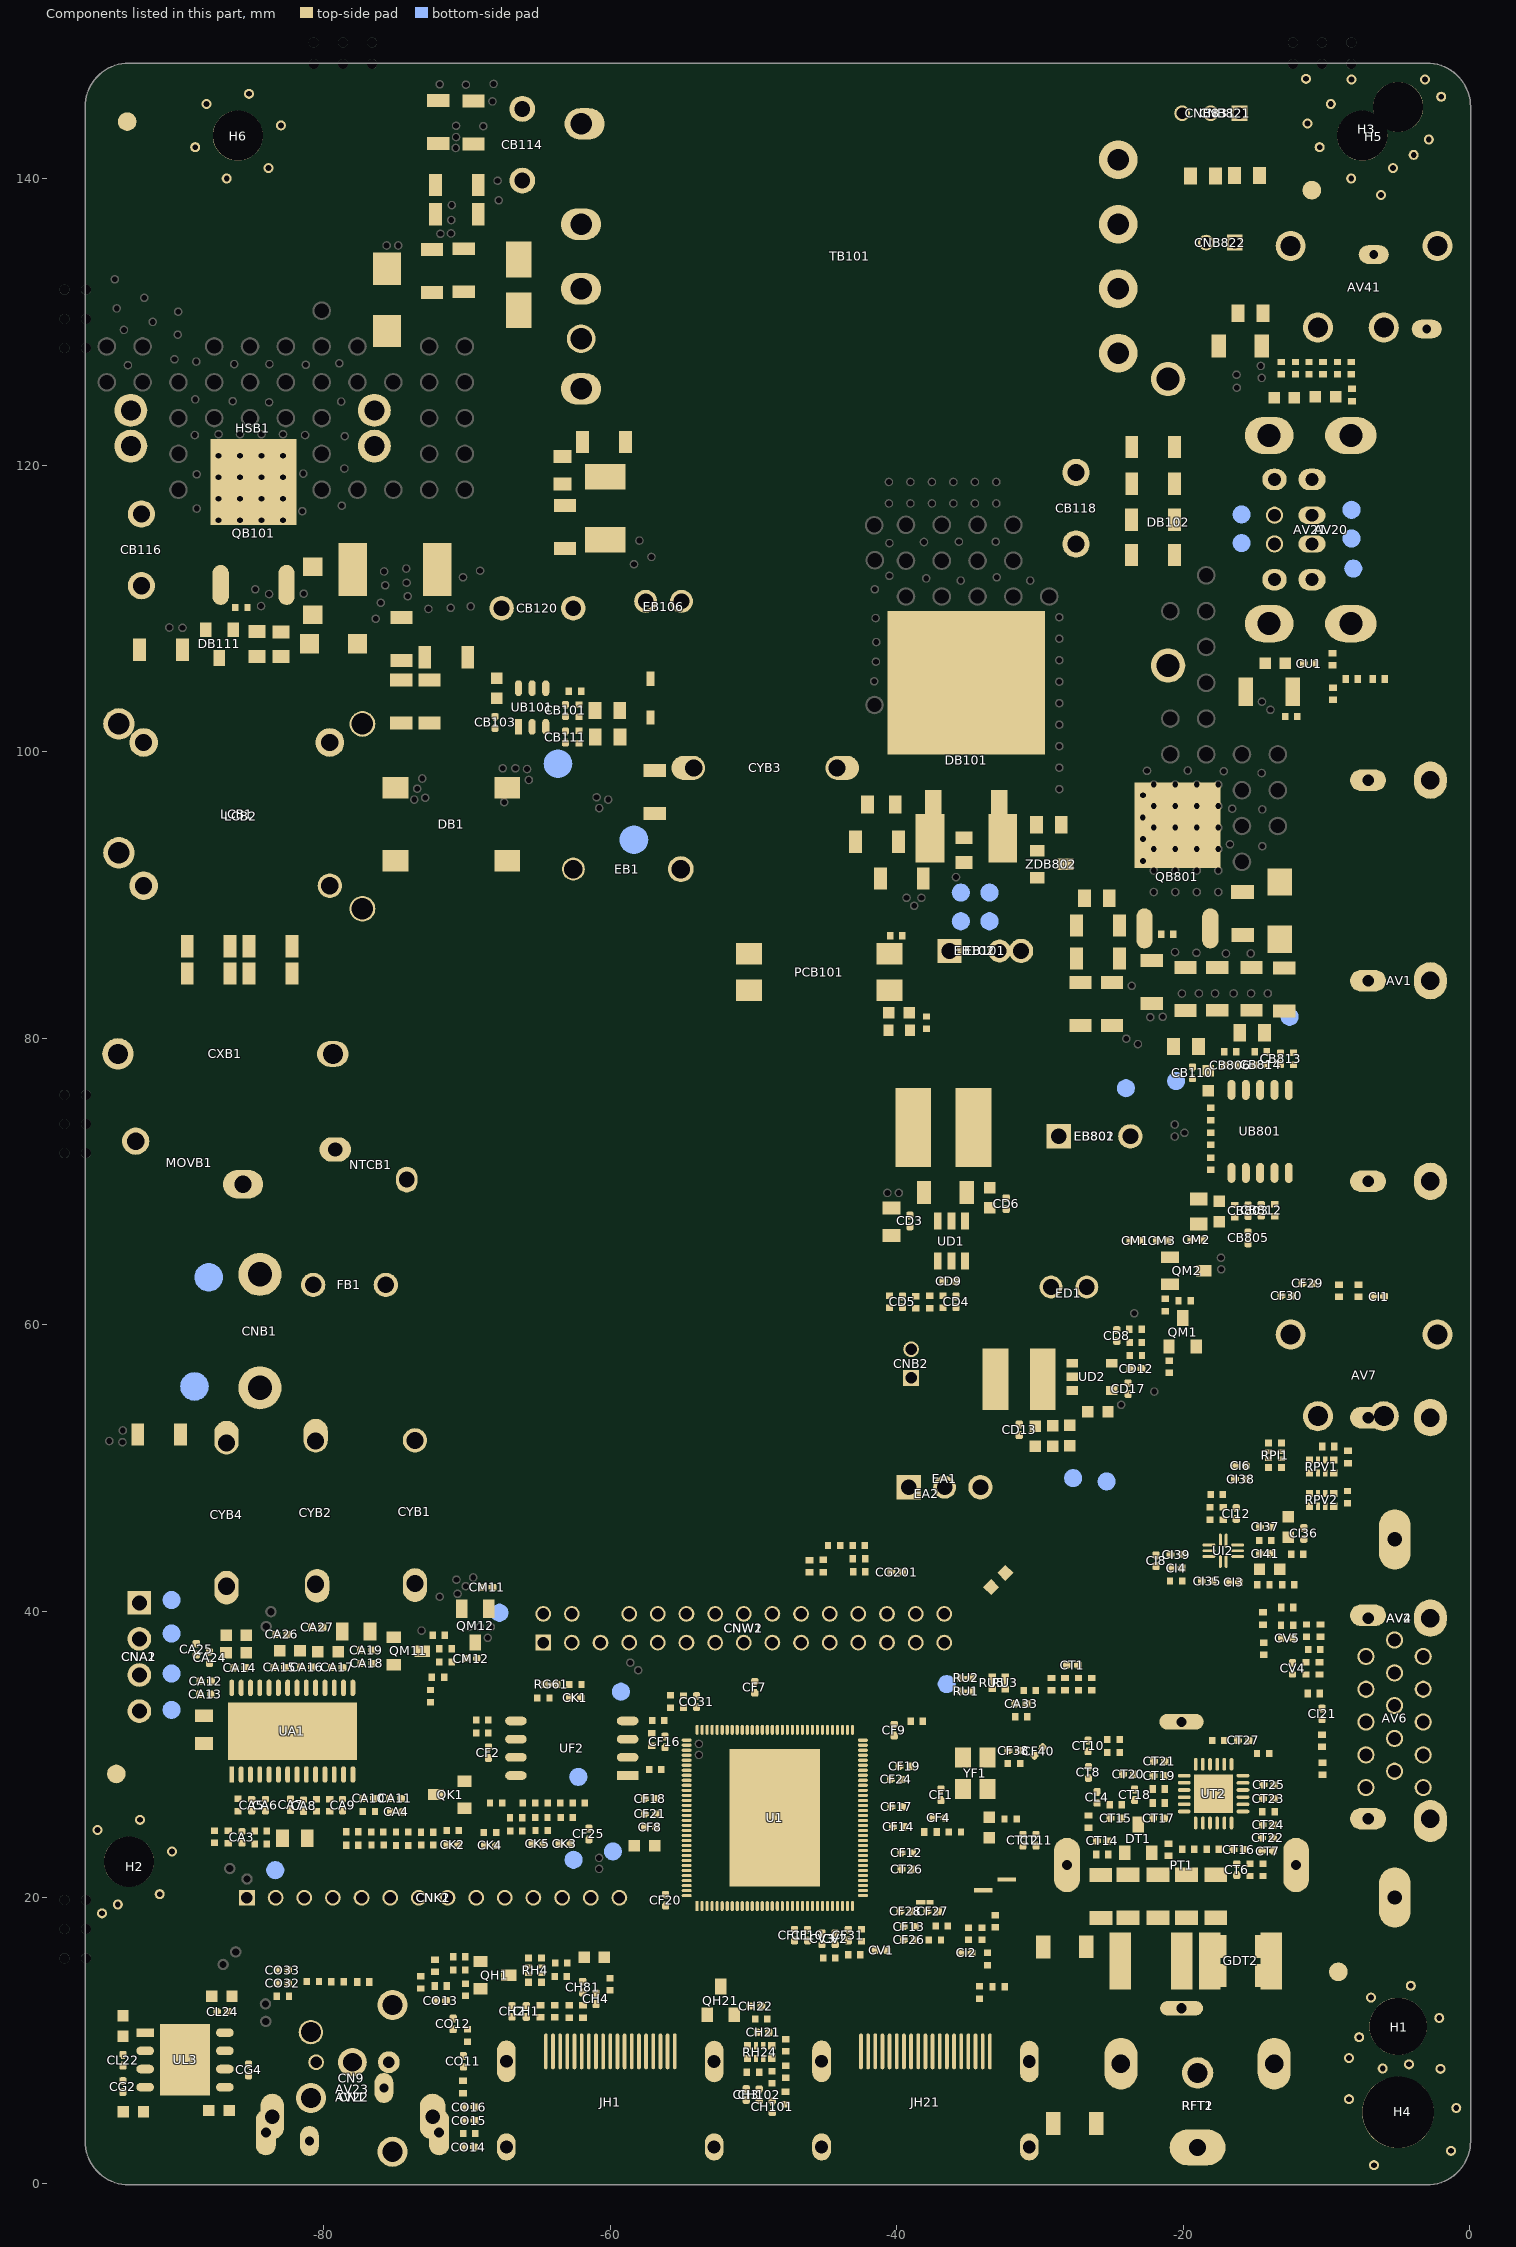
[diagram p0: the components of this part, seen from the top]
# Altium PCB MISC86372.PcbDoc (part 16 of 16)
Units mm, origin at the board's own origin, x right, y up, seen from the top; angles counter-clockwise.
Board outline 96.73 x 148.13 mm, 2 copper layers (TopLayer, BottomLayer), stack 1.571 mm thick; 578 components, 318 nets, 2702 pads, 836 vias.

## Silkscreen, mask and mechanical layers (free items; w line width, h text height)
TopOverlay:
  drawing of 502 lines, arcs and shapes, not listed
  text "2" at -3.2,226.609 h4.06
  text "3" at -191.5,220.391 h4.06 r180
  text "Solder Mask:" at 150.475,177.774 h1.52
  text "IPC SM-840" at 160.952,177.749 h1.52
  text "Silkscreen Color:" at 180.409,177.749 h1.52
  text "White" at 192.575,177.749 h1.52
  text "Units:" at 180.409,175.234 h1.52
  text "PTH Copper Thickness:" at 150.475,175.209 h1.52
  text ">20um" at 167.582,175.184 h1.52
  text "mm" at 185.438,175.196 h1.52
  text "Dielectric Constant Er@1GHz To 1MHz:" at 150.466,172.695 h1.52
  text "4.2 --- 4.6" at 180.425,172.708 h1.52
  text "Panel Size:" at 150.424,170.193 h1.52
  text "2L,4,97.35×148.75mm,FR4(TG130-CTI175),1OZ,Green,OSP,1.2mm" at 158.175,170.193 h1.52
  text "Silkscreen on PTH:" at 150.437,167.614 h1.52
  text "Primary Side Retained;" at 163.594,167.589 h1.52
  text "Secondary Side  Removed for Soldering" at 180.409,167.551 h1.52
  text "Special Requirements" at 150.411,165.311 h1.52
  text "If engineering questions are not answered within 2 hours, call PHONE_A" at 198.332,165.126 h1.52
  text "1. Lead-free HASL (HAL_LF, Lead Free Hot Air Leveling)" at 165.42,162.68 h1.52
  text "2. OSP (OSP, Organic Solderability Preservatives)" at 165.42,160.546 h1.52
  text "3. ENIG (ENIG, Electroless Nickel/Immersion Gold)" at 165.382,158.222 h1.52
  text "Plated Technics" at 152.316,157.34 h1.52
  text "4. ENIG + gold finger (ENIG_G/F, Electroless Nickel/Immersion Gold + Gold Finger)" at 165.42,156.178 h1.52
  text "5. Gold plating (Gold_plated, Gold-plated)" at 165.445,154.133 h1.52
  text "6. Gold plating + gold finger (Gold_Plated_G/F, Gold-plated + Gold Finger)" at 165.458,152.152 h1.52
  text "LED DRIVER" at -30.785,146.634 h1.52
  text "Impedance Control" at 150.532,146.345 h1.52
  text "Target Impedance" at 170.771,146.348 h1.52
  text "Layer(s)" at 209.23,146.35 h1.52
  text "Width & Clearance" at 189.715,146.342 h1.52
  text "75 +/- 10% Ohm" at 171.335,143.79 h1.52
  text "G/12/15.8/12/G mil" at 188.634,143.773 h1.52
  text "layer 1" at 209.23,143.776 h1.52
  text "Single End Impedance" at 150.532,142.616 h1.52
  text "75 +/- 10% Ohm" at 171.335,141.301 h1.52
  text "G/6.2/7.1/6.2/G mil" at 188.634,141.284 h1.52
  text "layer 1&2" at 209.23,141.287 h1.52
  text "[ Zo ]" at 156.208,139.13 h1.52
  text "G/5/7/5/7/5/G mil" at 188.888,133.841 h1.52
  text "100 +/- 10% Ohm" at 171.005,133.816 h1.52
  text "layer 1" at 209.509,133.771 h1.52
  text "Differential Impedance" at 150.528,132.416 h1.52
  text "9/4/9 mil" at 188.838,131.322 h1.52
  text "100 +/- 10% Ohm" at 170.955,131.297 h1.52
  text "layer 1" at 209.46,131.251 h1.52
  text "[ Zo ]" at 156.196,129.283 h1.52
  text "( G: Ground )" at 153.912,126.553 h1.52
  text "90 +/- 10% Ohm" at 171.666,126.247 h1.52
  text "layer 1" at 209.408,126.227 h1.52
  text "G/5/11/5/11/5/G mil" at 188.888,126.158 h1.52
  text "Common Mode Impedance" at 150.014,120.922 h1.52
  text "[ Zc ]" at 156.314,118.865 h1.52
  text "Refer to Gerber documents GTP&GBP for Stencil aperture design" at 173.257,112.154 h1.52
  text "Stencil" at 150.377,109.69 h1.52
  text "NEW" at 173.203,107.213 h1.52
  text "Test jig" at 150.329,104.721 h1.52
  text "The Same As XXXXXXXXXXXXXX XXXXXX" at 173.234,104.696 h1.52
  text "Wave-soldering jig" at 150.385,102.226 h1.52
  text "The Same As XXXXXXXXXXXXXX XXXXXX" at 173.285,102.055 h1.52
  text "Solder paste" at 173.194,99.64 h1.52
  text "Production process" at 150.346,99.602 h1.52
  text "[Process and notes]" at 154.924,97.447 h1.52
  text "Stencil at HDMI is cut to the actual pattern" at 173.304,97.409 h1.52
  text "Only one barcode position on the board; the other barcode must be attached to a component" at 192.075,97.409 h1.52
  text "Special requirements" at 150.372,94.573 h1.52
  text "SMD components over 2mm high on the wave-soldering side" at 150.365,91.999 h1.52
  text "Packaging notes" at 150.356,89.555 h1.52
  text "[Fragile components]" at 156.486,87.402 h1.52
  text "Footprint matching" at 150.356,84.475 h1.52
  text "[New component footprint]" at 156.13,82.347 h1.52
  text "(Automated Testing Support)" at 158.442,79.439 h1.14
  text "Automated test support" at 150.352,79.35 h1.52
  text "NO" at 174.919,78.064 h1.52
  text "[Reserved suction cup and press bar positions]" at 154.429,77.204 h1.52
  text "1" at -3.168,77.109 h4.06
  text "4" at -191.5,70.891 h4.06 r180
  text "Layer Stack Up Detail for" at 153.936,68.072 h2.54
  text ".Pcb_File_Name_No_Path" at 180.881,68.072 h2.54
  text "Layer" at 158.111,64.319 h1.27
  text "Gerber" at 167.552,64.319 h1.27
  text "Layer" at 175.455,64.319 h1.27
  text "Layer" at 191.616,64.319 h1.27
  text "Copper" at 211.654,64.319 h1.27
  text "Dielectric" at 219.573,64.319 h1.27
  text "Stack up" at 191.616,63.027 h1.27
  text "Height" at 219.573,63.027 h1.27
  text "Name" at 158.111,62.989 h1.27
  text "Document" at 167.552,62.989 h1.27
  text "Ordor" at 175.455,62.989 h1.27
  text "Thickness" at 211.654,62.989 h1.27
  text "12V" at -34.679,58.546 h1.27 r90
  text "TopOverlay" at 158.103,57.074 h1.52
  text ".GTO" at 168.506,57.009 h1.52
  text "PWR UPGRADE" at -41.614,56.411 h1.52 r90
  text "GND" at -34.699,54.948 h1.27 r90
  text "0.4mil" at 219.505,54.85 h1.52
  text "1" at 176.807,52.23 h1.52
  text "1.4mil" at 211.986,52.228 h1.52
  text "2" at 176.808,46.818 h1.52
  text "1.4mil" at 211.942,46.793 h1.52
  text "0.4mil" at 219.573,44.388 h1.52
  text "LVDS" at -61.109,42.924 h1.52
  text "Notes:" at 149.768,30.091 h2.03
  text "1. No Plated Through Hole  overlap each other should be combined ,Residues between them should be eliminated." at 149.746,27.858 h1.52
  text "SPEAKER" at -93.142,26.797 h1.52
  text "2. Plated Through Hole superposition should be made as a bigger one." at 149.745,25.925 h1.52
  text "3. When there is not enough space for UL authentication marking,Manufacturer ID code and the Bar Code frame," at 149.746,24.185 h1.52
  text "only the Manufacturer  ID code is needed and layed wherever it can be." at 151.229,22.39 h1.52
  text "4. Spacing between two pads of IC package should be covered with solder oil." at 149.746,20.44 h1.52
  text "5. All trace should be covered with green oil unless otherwise specified. If discovers unusually, please confirm with us." at 149.746,18.575 h1.52
  text "KEY&IR&LED" at -88.468,17.704 h1.52 r90
  text "6. Silkscreen overlaped SMD pads should be removed directly." at 149.746,16.713 h1.52
  text "7. The width of Carbon Sprayed must be 16mil wider than its trace." at 149.746,14.909 h1.52
  text "8. Bridging Thickness of V-cut  should be kept within 0.3±0.1mm when the width of single piece bare board is smaller than 20mm." at 149.746,13.018 h1.52
  text "9. There is no need to plugged with green oil when the diameter of vias is bigger than 0.6mm." at 149.746,10.94 h1.52
  text "10. All vias under BGA must be covered and plugged with Solder oil." at 149.747,8.911 h1.52
BottomOverlay:
  drawing of 153 lines, arcs and shapes, not listed
  text "+" at -15.697,146.069 h2
  text "-" at -19.676,145.949 h3
  text "-" at -17.676,145.949 h3
  text "EARPHONE OUT" at -1.064,137.184 h1.52
  text "+" at -15.799,137.135 h2
  text "-" at -17.907,137.008 h3
  text "USB2 IN" at -3.967,111.681 h1.52 r270
  text "USB1 IN" at -1.986,111.656 h1.52 r270
  text "AV IN / YPBPR AUDIO IN" at -5.436,69.723 h1.52 r270
  text "FB1" at -71.501,59.766 h1.27
  text "PC AUDIO IN" at -1.408,56.142 h1.52
  text ".GBO" at 168.547,41.934 h1.52
  text "BottomOverlay" at 157.837,41.909 h1.52
  text "VGA IN" at -2.393,18.128 h1.52 r270
  text "K7" at -83.795,17.018 h1.27 r270
  text "K6" at -81.661,17.018 h1.27 r270
  text "K5" at -79.681,17.018 h1.27 r270
  text "K4" at -77.755,17.018 h1.27 r270
  text "K3" at -75.717,17.018 h1.27 r270
  text "K2" at -73.681,17.018 h1.27 r270
  text "K1" at -71.653,17.018 h1.27 r270
  text "K0" at -69.647,17.018 h1.27 r270
  text "YPBPR IN" at -8.623,16.897 h1.52 r270
  text "IR" at -65.684,16.79 h1.27 r270
  text "5V" at -59.512,16.637 h1.27 r270
  text "RED" at -61.758,16.129 h1.27 r270
  text "GND" at -67.742,16.027 h1.27 r270
  text "GRN" at -63.729,16.027 h1.27 r270
  text "GND" at -85.979,15.977 h1.27 r270
  text "MINIAV OUT" at -73.076,15.443 h1.52
  text "OPTICAL OUT" at -72.796,14.173 h1.52
  text "RF IN" at -12.733,2.59 h1.52
  text "HDMI2 IN" at -34.77,0.796 h1.52
  text "HDMI1(ARC) IN" at -54.844,0.732 h1.52
  text "COAX/CVBS OUT" at -76.886,0.616 h1.52
TopPaste:
  rectangle: -31.349,4.458 -29.835,5.461
  rectangle: 153.901,58.987 157.208,60.987
  rectangle: -29.184,0.309 -28.94,3.2
  rectangle: -31.342,3.099 -29.82,4.064
  region: -31.342,5.309
  region: -31.342,5.309
  region: -31.349,4.458 -31.346,9.887 -29.116,9.892 -29.116,5.369 -29.83,5.369 -29.83,4.458
  region: -31.333,4.075 -31.3,4.041 -29.852,4.041 -29.852,3.173 -29.857,3.169 -29.851,3.163 -29.156,3.163 -29.156,0.298 -29.162,0.303 -31.327,0.303 -31.327,4.049 -31.342,4.064
  lines w0.127: 167.894,58.987 167.894,60.987 ; 153.901,58.987 172.494,58.987 172.494,60.987 153.901,60.987 153.901,58.987
  lines w0.8: -65.735,93.548 -63.297,95.987
  text "TopPaste" at 158.103,59.526 h1.52
  text ".GTP" at 168.506,59.472 h1.52
BottomPaste:
  rectangle: 153.901,38.983 157.208,40.983
  lines w0.127: 167.894,38.983 167.894,40.983 ; 153.901,38.983 172.494,38.983 172.494,40.983 153.901,40.983 153.901,38.983
  text "BottomPaste" at 157.782,39.567 h1.52
  text ".GBP" at 168.529,39.437 h1.52
TopSolder:
  rectangle: 153.901,54.162 157.208,56.162
  region: -75.87,9.017 -76.302,8.585 -76.302,6.695 -75.982,6.375 -74.905,7.453 -74.905,8.883
  lines w0.127: 167.894,54.162 167.894,56.162 ; 153.901,54.162 172.494,54.162 172.494,56.162 153.901,56.162 153.901,54.162
  lines w0.8: -65.735,93.548 -63.297,95.987
  text "TopSolder" at 158.116,54.673 h1.52
  text ".GTS" at 168.506,54.631 h1.52
BottomSolder:
  drawing of 44 lines, arcs and shapes, not listed
  text "BottomSolder" at 157.782,44.302 h1.52
  text ".GBS" at 168.505,44.279 h1.52
过炉治具:
  drawing of 291 lines, arcs and shapes, not listed
3D和装配:
  circle w0.127: c-9.474,57.988 r15
  circle w0.254: c-24.384,33.246 r25
  circle w0.254: c-8.585,69.977 r25
  circle w0.127: c-7.1,70 r15
  circle w0.127: c-27.4,37.504 r15
  lines w0.127: -5.5,-5.207 -5.5,145 ; -66.747,0.785 -53.247,0.785 -53.247,14.285 -66.747,14.285 -66.747,0.785 ; -44.747,0.785 -31.247,0.785 -31.247,14.285 -44.747,14.285 -44.747,0.785
  text "2L,4,97.35×148.75mm,FR4(TG130-CTI175),1OZ,Green,OSP,1.2mm,5,80,89.4%,1858,0.4mm" at 158.175,170.193 h1.52
自动测试:
  circle w0.152: c-47.409,108.128 r5
  circle w0.152: c-47.38,108.128 r6
  circle w0.152: c-90.179,134.366 r6
  circle w0.152: c-90.208,134.366 r5
顶层限制:
  drawing of 1339 lines, arcs and shapes, not listed
  text "100" at -49.698,167.75 h2.5
  text "89" at -44.198,163.25 h2.5
  text "86" at -42.698,158.75 h2.5
  text "7.5" at -12.856,154.25 h2.5
  text "5" at -2.198,149.75 h2.5
  text "LED DRIVER}" at -51.749,137.101 h3
  text "4-3.5" at -101.544,133.144 h2.5
  text "14" at 11.698,89.217 h2.5 r90
  text "Minimise board expansion}" at -131.258,87.307 h3
  text "14" at 11.743,75.217 h2.5 r90
  text "148" at 51.683,72.75 h2.5 r90
  text "145" at 47.183,71.25 h2.5 r90
  text "143" at 42.683,70.25 h2.5 r90
  text "AC IN}" at -83.133,65.664 h3
  text "132.5" at 38.183,65 h2.5 r90
  text "115.5" at 33.683,56.5 h2.5 r90
  text "LVDS}" at -54.23,46.212 h3
  text "14" at 11.698,44.717 h2.5 r90
  text "84" at 29.183,40.75 h2.5 r90
  text "SPEAKER}" at -88.497,36.189 h3
  text "73.25" at -108.379,35.375 h2.5 r90
  text "14" at 11.743,30.717 h2.5 r90
  text "56.5" at 24.683,27 h2.5 r90
  text "IR&KEY}" at -78.542,24.614 h3
  text "5.2" at 11.19,23.327 h2.5 r90
  text "39.5" at 20.183,18.5 h2.5 r90
  text "4" at -18.265,16.421 h2.5
  text "32.5" at 15.683,15 h2.5 r90
  text "22.5" at -103.241,13.522 h2.5 r90
  text "5" at -20.379,12.074 h2.5
  text "11" at 11.183,4.25 h2.5 r90
  text "5" at 6.683,1.25 h2.5 r90
  text "5" at -2.5,-11.073 h2.5
  text "19" at -9.5,-15.573 h2.5
  text "38" at -19,-20.073 h2.5
  text "60" at -30,-24.573 h2.5
  text "78" at -39,-29.073 h2.5
  text "93.6" at -46.8,-33.573 h2.5
  text "96.6" at -48.3,-38.073 h2.5
  text "100" at -50,-42.573 h2.5
附加说明:
  region: -98.1,21.083 -96.6,21.083 -96.6,14.503 -98.1,14.503 hole: -97.35,17.509 -97.634,17.793 -97.35,18.078 -97.066,17.793
  region: -98.1,77.29 -96.6,77.29 -96.6,70.71 -98.1,70.71 hole: -97.35,73.716 -97.634,74 -97.35,74.284 -97.066,74
  region: -96.6,126.917 -98.1,126.917 -98.1,133.497 -96.6,133.497 hole: -97.35,130.491 -97.066,130.207 -97.35,129.922 -97.634,130.207
  region: -96.597,276.417 -98.097,276.417 -98.097,282.997 -96.597,282.997 hole: -97.347,279.991 -97.063,279.707 -97.347,279.422 -97.632,279.707
  region: -98.097,226.79 -96.597,226.79 -96.597,220.21 -98.097,220.21 hole: -97.347,223.216 -97.632,223.5 -97.347,223.784 -97.063,223.5
  region: -98.097,170.583 -96.597,170.583 -96.597,164.003 -98.097,164.003 hole: -97.347,167.009 -97.632,167.293 -97.347,167.578 -97.063,167.293
  region: -75.372,149.5 -75.372,148 -81.952,148 -81.952,149.5 hole: -78.946,148.75 -78.662,149.034 -78.378,148.75 -78.662,148.466
  region: -7.015,149.5 -7.015,148 -13.595,148 -13.595,149.5 hole: -10.589,148.75 -10.305,149.034 -10.02,148.75 -10.305,148.466
  region: -119.63,148 -119.63,149.5 -113.05,149.5 -113.05,148 hole: -116.056,148.75 -116.34,148.466 -116.624,148.75 -116.34,149.034
  region: -187.987,148 -187.987,149.5 -181.407,149.5 -181.407,148 hole: -184.413,148.75 -184.697,148.466 -184.982,148.75 -184.697,149.034
  lines w0.127: 257.353,165.934 286.055,165.934 ; 257.353,168.66 286.055,168.66 ; 257.353,171.387 286.055,171.387 ; 257.353,174.113 286.055,174.113 ; 257.353,176.839 293.688,176.839 ; 264.986,163.208 264.986,179.565 ; 286.055,163.208 286.055,179.565 ; 257.353,163.208 293.688,163.208 293.688,179.565 257.353,179.565 257.353,163.208
  text "Template date:" at 201.571,177.737 h1.52
  text "Version cycle number" at 257.908,177.707 h1.52
  text "PCB designer" at 272.018,177.695 h1.52
  text "Customer" at 288.858,177.707 h1.52
  text "2018.12.27" at 209.75,177.648 h1.52
  text "Board material utilisation:" at 201.558,175.273 h1.52
  text "8X%" at 209.75,175.171 h1.52
  text "(Fill in for non-TV division projects)" at 214.576,175.171 h1.52
  text "XXXXXX" at 258.403,174.989 h1.52
  text "HYW" at 266.125,174.968 h1.52
  text "XXXXXX" at 258.403,172.322 h1.52
  text "HYW" at 266.176,172.174 h1.52
  text "XXXXXX" at 258.327,169.757 h1.52
  text "HYW" at 266.277,169.66 h1.52
  text "COMPANY_A" at 287.055,169.647 h1.52
  text "XXXXXX" at 258.327,167.039 h1.52
  text "HYW" at 266.277,166.942 h1.52
  text "Special requirements; leave blank if none" at 165.761,165.096 h1.52
  text "The notes below must be copied to the TopOverlay layer; one or two items may be noted" at 191.093,99.543 h1.52
  text "SMD components 3.5mm from PCB clamping edge; production must control specially" at 173.186,97.46 h1.52
  text "No barcode position on the board; barcode must be attached to a component" at 229.667,97.458 h1.52
  text "Customer special requirements; special process requirements; leave blank if none" at 173.137,94.591 h1.52
  text "Height value and reference designator of SMD components over 2mm on the solder side; leave blank if none" at 173.137,92.051 h1.52
  text "Reference designators of fragile components; leave blank if none" at 173.092,88.339 h1.52
  text "Reference designators of new footprints; leave blank if none" at 173.152,83.08 h1.52
  text "Suction cup and press bar positions reserved: fill 'Yes', otherwise 'No'" at 173.174,77.928 h1.52
  text "X.XXXX.XXX Stencil Revision Explanation" at 149.622,6.3 h1.52
  text "X.XXXX.XXX Testing jig Revision Explanation" at 149.61,4.548 h1.52
  text "X.XXXX.XXX Wave-soldering jig Revision Explanation" at 149.597,2.821 h1.52
DrillDrawing:
  text ".Legend" at 149.827,180.79 h1.52